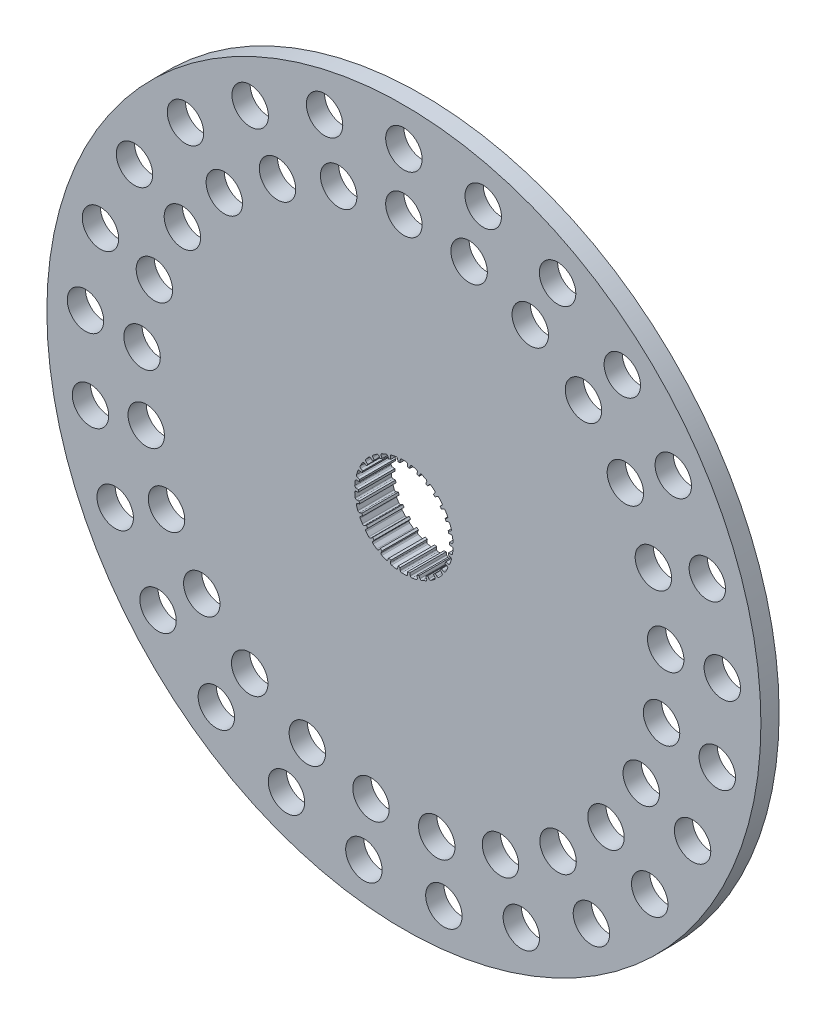
from build123d import *

# Parameters (mm, degrees)
SKETCH1_R           = 98
BOSS_EXTRUDE1_DEPTH = 5
SKETCH2_R           = 5
CUT_EXTRUDE1_DEPTH  = 5
SKETCH4_R           = 40.197144264
SKETCH3_R           = 60.197144264
SKETCH5_R           = 12.5
CUT_EXTRUDE2_DEPTH  = 139.953229541
CUT_EXTRUDE3_DEPTH  = 139.953229541
CIRPATTERN1_COUNT   = 30


with BuildPart() as part:
    # Sketch1 → Boss-Extrude1 (new body)
    with BuildSketch(Plane.XY):
        Circle(SKETCH1_R)
    extrude(amount=BOSS_EXTRUDE1_DEPTH)

    # Sketch2 → Cut-Extrude1 (cut)
    with BuildSketch(Plane.XY.offset(5)):
        with Locations((0, 87.574842429)):
            Circle(SKETCH2_R)
        with Locations((21.778977682, 84.823517715)):
            Circle(SKETCH2_R)
        with Locations((42.189502099, 76.742419424)):
            Circle(SKETCH2_R)
        with Locations((59.949104937, 63.839312682)):
            Circle(SKETCH2_R)
        with Locations((73.941885034, 46.924947139)):
            Circle(SKETCH2_R)
        with Locations((83.288624555, 27.06211459)):
            Circle(SKETCH2_R)
        with Locations((87.402033482, 5.498869854)):
            Circle(SKETCH2_R)
        with Locations((86.023651202, -16.409889099)):
            Circle(SKETCH2_R)
        with Locations((79.240086545, -37.287554368)):
            Circle(SKETCH2_R)
        with Locations((67.477575825, -55.822305462)):
            Circle(SKETCH2_R)
        with Locations((51.475200851, -70.849535804)):
            Circle(SKETCH2_R)
        with Locations((32.238449695, -81.425029245)):
            Circle(SKETCH2_R)
        with Locations((10.976038181, -86.884288639)):
            Circle(SKETCH2_R)
        with Locations((-10.97603818, -86.884288639)):
            Circle(SKETCH2_R)
        with Locations((-32.238449695, -81.425029245)):
            Circle(SKETCH2_R)
        with Locations((-51.475200851, -70.849535804)):
            Circle(SKETCH2_R)
        with Locations((-67.477575825, -55.822305462)):
            Circle(SKETCH2_R)
        with Locations((-79.240086545, -37.287554368)):
            Circle(SKETCH2_R)
        with Locations((-86.023651202, -16.409889099)):
            Circle(SKETCH2_R)
        with Locations((-87.402033482, 5.498869854)):
            Circle(SKETCH2_R)
        with Locations((-83.288624555, 27.06211459)):
            Circle(SKETCH2_R)
        with Locations((-73.941885034, 46.924947139)):
            Circle(SKETCH2_R)
        with Locations((-59.949104937, 63.839312682)):
            Circle(SKETCH2_R)
        with Locations((-42.189502099, 76.742419424)):
            Circle(SKETCH2_R)
        with Locations((-21.778977682, 84.823517715)):
            Circle(SKETCH2_R)
        with Locations((0, 72)):
            Circle(SKETCH2_R)
        with Locations((17.905671876, 69.737987601)):
            Circle(SKETCH2_R)
        with Locations((34.686264535, 63.094080963)):
            Circle(SKETCH2_R)
        with Locations((49.287391627, 52.485741174)):
            Circle(SKETCH2_R)
        with Locations((60.791610636, 38.579529238)):
            Circle(SKETCH2_R)
        with Locations((68.476069173, 22.249223595)):
            Circle(SKETCH2_R)
        with Locations((71.857924447, 4.520917406)):
            Circle(SKETCH2_R)
        with Locations((70.724682052, -13.49145465)):
            Circle(SKETCH2_R)
        with Locations((65.147547778, -30.656108993)):
            Circle(SKETCH2_R)
        with Locations((55.47695348, -45.894527262)):
            Circle(SKETCH2_R)
        with Locations((42.320538165, -58.249223595)):
            Circle(SKETCH2_R)
        with Locations((26.504967793, -66.943906984)):
            Circle(SKETCH2_R)
        with Locations((9.023992817, -71.432258495)):
            Circle(SKETCH2_R)
        with Locations((-9.023992817, -71.432258495)):
            Circle(SKETCH2_R)
        with Locations((-26.504967793, -66.943906984)):
            Circle(SKETCH2_R)
        with Locations((-42.320538165, -58.249223595)):
            Circle(SKETCH2_R)
        with Locations((-55.47695348, -45.894527262)):
            Circle(SKETCH2_R)
        with Locations((-65.147547778, -30.656108993)):
            Circle(SKETCH2_R)
        with Locations((-70.724682052, -13.49145465)):
            Circle(SKETCH2_R)
        with Locations((-71.857924447, 4.520917406)):
            Circle(SKETCH2_R)
        with Locations((-68.476069173, 22.249223595)):
            Circle(SKETCH2_R)
        with Locations((-60.791610636, 38.579529238)):
            Circle(SKETCH2_R)
        with Locations((-49.287391627, 52.485741174)):
            Circle(SKETCH2_R)
        with Locations((-34.686264535, 63.094080963)):
            Circle(SKETCH2_R)
        with Locations((-17.905671876, 69.737987601)):
            Circle(SKETCH2_R)
    extrude(amount=-CUT_EXTRUDE1_DEPTH, mode=Mode.SUBTRACT)

    # Sketch4 → Loft1 section 0
    with BuildSketch(Plane(origin=(0, 0, -5), x_dir=(-1, 0, 0), z_dir=(0, 0, -1))):
        Circle(SKETCH4_R)
    # Sketch3 → Loft1 section 1
    with BuildSketch(Plane(origin=(0, 0, 0), x_dir=(-1, 0, 0), z_dir=(0, 0, -1))):
        Circle(SKETCH3_R)
    loft()

    # Sketch5 → Cut-Extrude2 (cut, through all)
    with BuildSketch(Plane(origin=(0, 0, -5), x_dir=(-1, 0, 0), z_dir=(0, 0, -1))):
        Circle(SKETCH5_R)
    extrude(amount=-CUT_EXTRUDE2_DEPTH, mode=Mode.SUBTRACT)

    # Sketch7 → Cut-Extrude3 (cut, through all)
    with BuildSketch(Plane(origin=(0, 0, -5), x_dir=(-1, 0, 0), z_dir=(0, 0, -1))):
        with BuildLine():
            Line((-0.6, 13.5), (0.6, 13.5))
            ThreePointArc((0.6, 13.5), (0.882842712, 13.382842712), (1, 13.1))
            Line((1, 13.1), (1, 11.5))
            Line((1, 11.5), (-1, 11.5))
            Line((-1, 11.5), (-1, 13.1))
            ThreePointArc((-1, 13.1), (-0.882842712, 13.382842712), (-0.6, 13.5))
        make_face()
    cut_extrude3 = extrude(amount=-CUT_EXTRUDE3_DEPTH, mode=Mode.SUBTRACT)

    # CirPattern1: Cut-Extrude3 ×30 about axis
    cirpattern1_axis = Axis((0, 0, 0), (0, 0, 1))
    for i in range(1, CIRPATTERN1_COUNT):
        add(cut_extrude3.rotate(cirpattern1_axis, i * 360 / CIRPATTERN1_COUNT), mode=Mode.SUBTRACT)


solid = part.part
